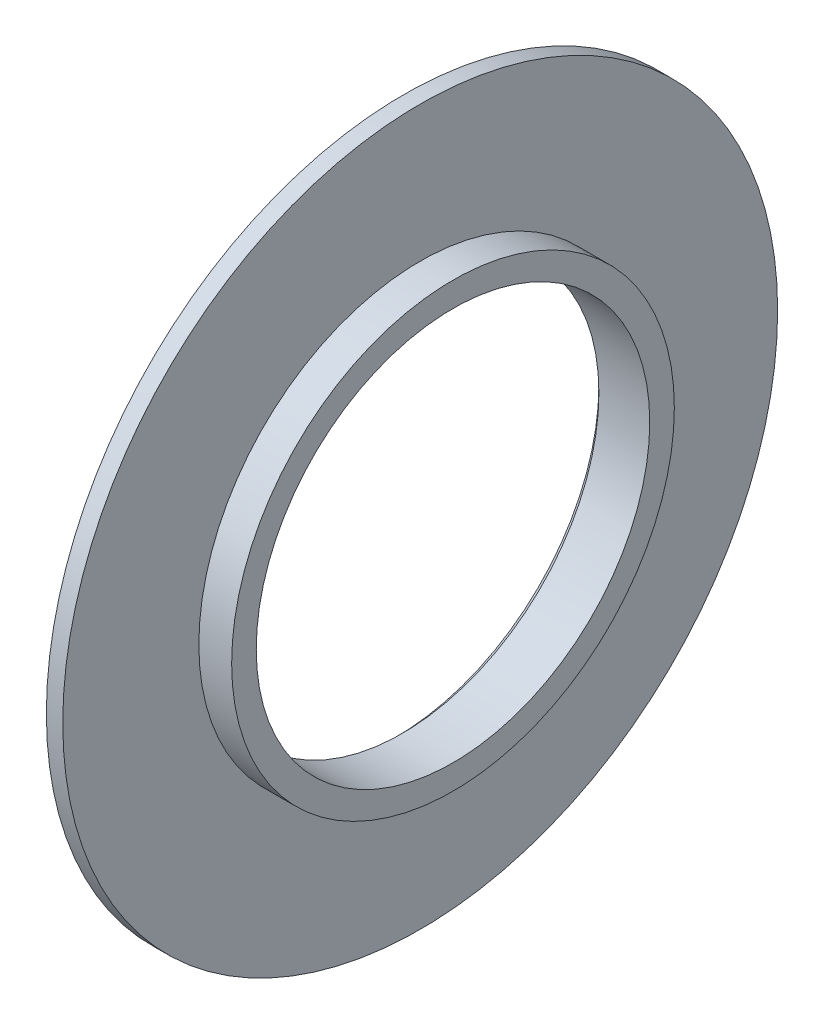
from build123d import *

# Parameters (mm, degrees)
CHAMFER1_SIZE = 4


with BuildPart() as part:
    # Sketch1 → Revolve1 (revolve)
    with BuildSketch(Plane.XY, mode=Mode.PRIVATE) as revolve1_sk:
        Polygon((0, 140), (5, 140), (5, 218), (15, 218), (15, 135), (35, 135), (35, 120), (0, 120), align=None)
    revolve(revolve1_sk.sketch.rotate(Axis((0, 0, 0), (1, 0, 0)), 90), axis=Axis((0, 0, 0), (1, 0, 0)))

    # Chamfer1
    chamfer1_edges = [part.edges().sort_by_distance(p)[0] for p in [
        (0, 0, -120),
    ]]
    chamfer(chamfer1_edges, length=CHAMFER1_SIZE)


solid = part.part
